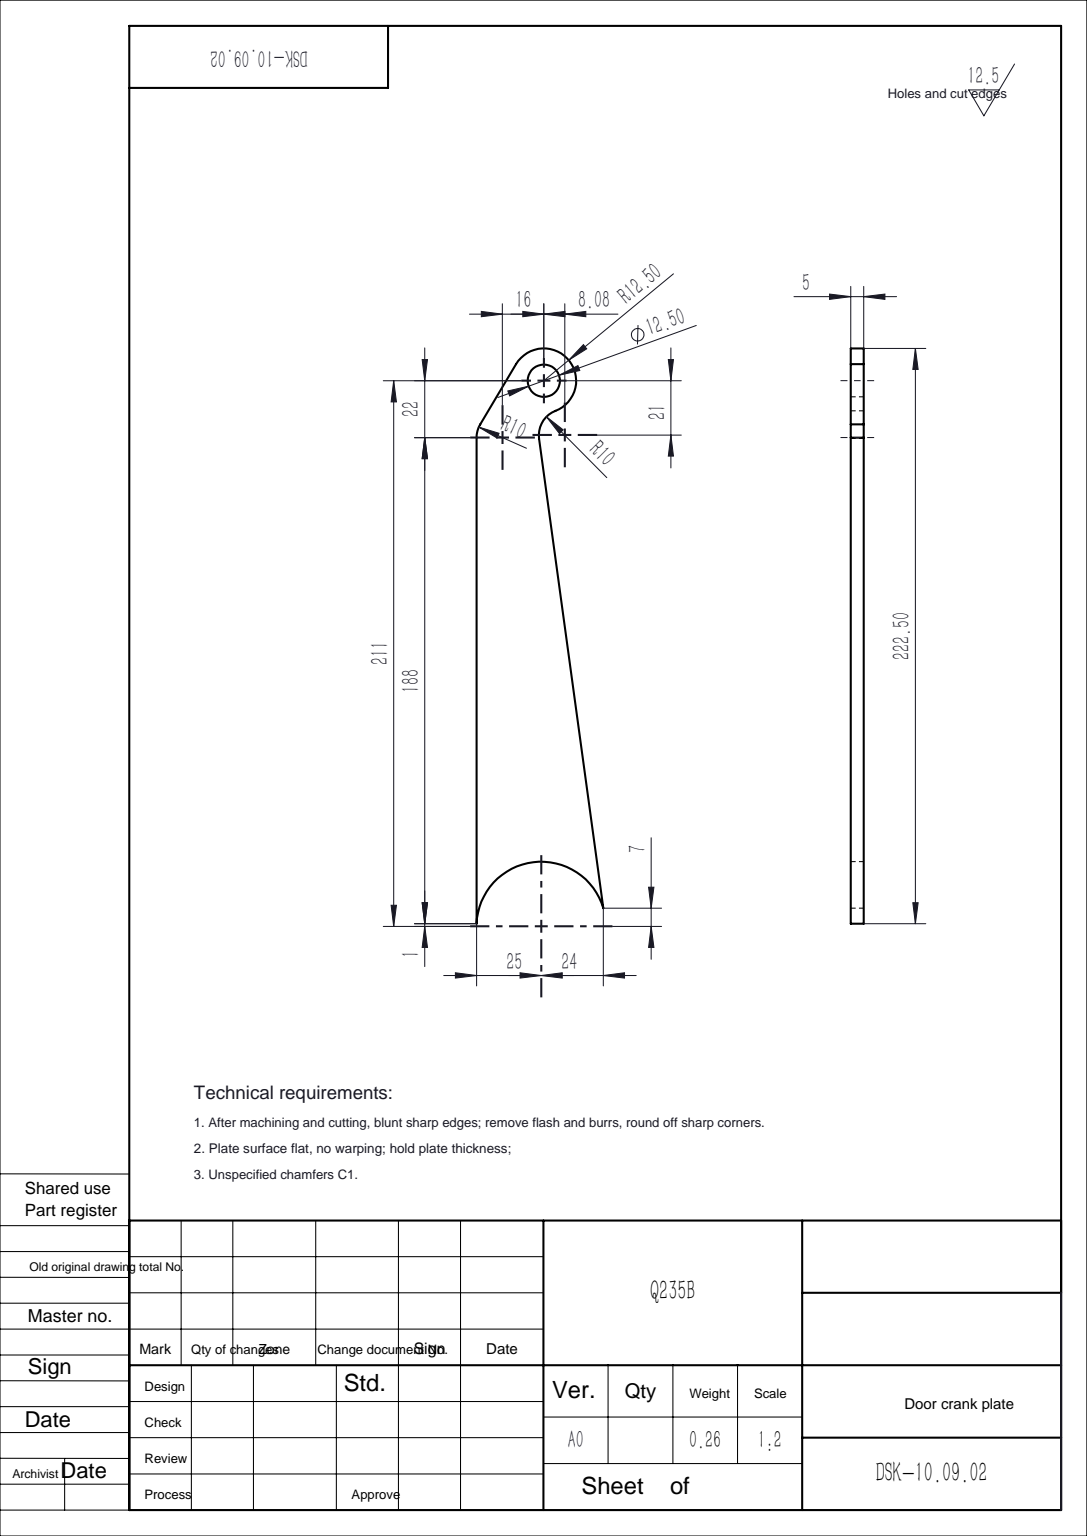
SolidWorks part; units mm, degrees
material "Q235B"
ref_plane "Front Plane" through (0, 0, 0) normal (0, 0, 1) x (1, 0, 0)
ref_plane "Top Plane" through (0, 0, 0) normal (0, 1, 0) x (1, 0, 0)
ref_plane "Right Plane" through (0, 0, 0) normal (1, 0, 0) x (0, 0, -1)
sketch "Sketch1" plane through (0, 0, 0) normal (0, 0, 1) x (1, 0, 0)
  line L0 (-25, 0) -> (25, 0) construction
  line L1 (-33.4221, 1) -> (25, 1) construction
  line L2 (-25, 1) -> (25, 1) construction
  line L3 (-24.98, 1) -> (-24.98, 189)
  line L4 (-25, 7) -> (24, 7) construction
  line L5 (24, 7) -> (-0.8103, 188.6467)
  line L6 (-23.5737, 194.1136) -> (-9.7221, 217.392)
  line L7 (-25, 7) -> (25, 7) construction
  circle A0 centre (0, 0) radius 25
  circle A1 centre (1.02, 211) radius 12.5
  arc A3 (-23.5737, 194.1136) -> (-24.98, 189) centre (-14.98, 189) ccw
  circle A4 centre (1.02, 211) radius 6.25
  arc A5 (5.5076, 199.3333) -> (-0.8103, 188.6467) centre (9.0978, 190) ccw
  dimension "D1" = 50
  dimension "D4" = 25
  dimension "D5" = 24
  dimension "D6" = 20
  dimension "D7" = 211
  dimension "D12" = 12.5
  dimension "D11" = 21
  dimension "D10" = 10
  dimension "D2" = 1
  dimension "D8" = 188
  dimension "D9" = 16
extrude "Boss-Extrude1" add sketch "Sketch1" along normal blind 5
